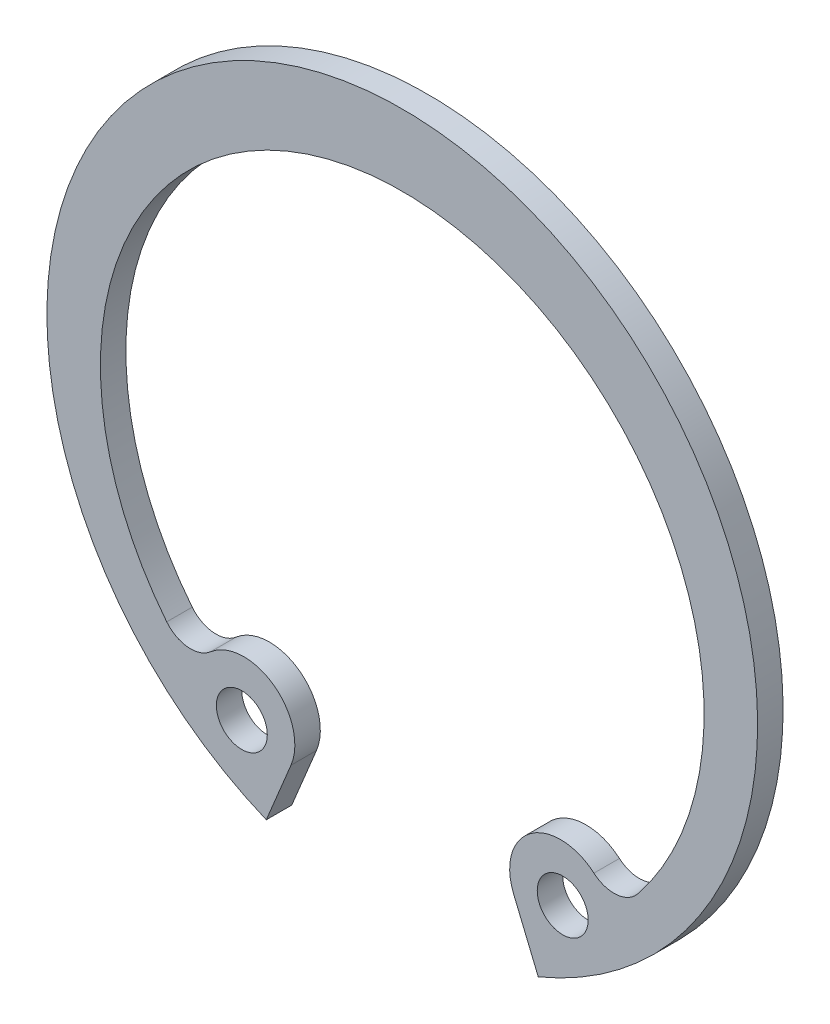
SolidWorks part; units mm, degrees
ref_plane "前视" through (0, 0, 0) normal (0, 0, 1) x (1, 0, 0)
ref_plane "上视" through (0, 0, 0) normal (0, 1, 0) x (1, 0, 0)
ref_plane "右视" through (0, 0, 0) normal (1, 0, 0) x (0, 0, -1)
sketch "尺寸草图" plane through (0, 0, 0) normal (0, 0, 1) x (1, 0, 0)
  line L0 (-13.95, 0) -> (13.95, 0) construction
  line L1 (0, 0) -> (-12.0811, -6.975) construction
  circle A0 centre (0, 0) radius 13.95
  point P5 (-9.75, 0)
  point P6 (10.6, 0)
  point P7 (2, 0)
  point P8 (11.8, 0)
  point P10 (-2.36, 0)
  point P11 (-0.7, 0)
  point P12 (-4.36, 0)
  point P13 (-10.95, 0)
  point P14 (26.8901, 15.525)
sketch "草图1" plane through (0, 0, 0) normal (0, 0, 1) x (1, 0, 0)
  line L0 (0, 13.95) -> (0, -12.8881) construction
  line L1 (-4.3688, -10.5471) -> (-5.3384, -12.8881)
  line L2 (-6.3797, -10.1756) -> (-6.2165, -9.7818) construction
  line L3 (0, 0) -> (-5.3384, -12.8881) construction
  line L4 (4.3688, -10.5471) -> (5.3384, -12.8881)
  arc A0 (5.3384, -12.8881) -> (-5.3384, -12.8881) centre (0, 0) ccw
  arc A1 (9.2459, -8.1118) -> (-9.2459, -8.1118) centre (0, -0.7) ccw
  circle A2 centre (-6.2981, -9.9787) radius 1
  arc A3 (-4.3688, -10.5471) -> (-7.5247, -8.2689) centre (-6.2165, -9.7818) ccw
  arc A4 (-7.5247, -8.2689) -> (-9.2459, -8.1118) centre (-8.3096, -7.3613) cw
  circle A5 centre (6.2981, -9.9787) radius 1
  arc A6 (4.3688, -10.5471) -> (7.5247, -8.2689) centre (6.2165, -9.7818) cw
  arc A7 (7.5247, -8.2689) -> (9.2459, -8.1118) centre (8.3096, -7.3613) ccw
extrude "基体-拉伸" add sketch "草图1" along normal blind 1
equation "\"D1@草图1\" = \"DD@尺寸草图\" "
equation "\"D2@草图1\"=\"d@尺寸草图\""
equation "\"D3@草图1\" = \"c@尺寸草图\""
equation "\"D6@草图1\" = \"RR@尺寸草图\""
equation "\"D8@草图1\" = \"R2@尺寸草图\""
equation "\"D7@草图1\" = \"R1@尺寸草图\""
equation "\"D4@草图1\" = \"aa@尺寸草图\"/2"
equation "\"D9@草图1\" = \"a@尺寸草图\""
equation "\"D5@草图1\" = \"d1@尺寸草图\""
equation "\"D1@基体-拉伸\" = \"s@尺寸草图\"/2"
equation "\"D2@基体-拉伸\" = \"D1@基体-拉伸\""
